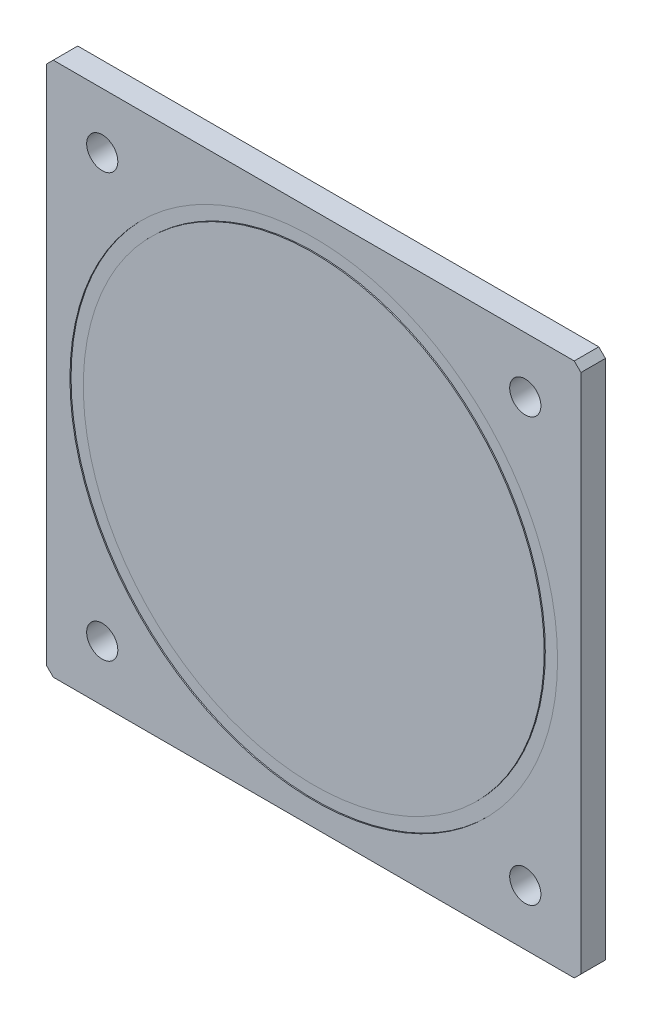
from build123d import *

# Parameters (mm, degrees)
SKETCH1_W           = 240
SKETCH1_H           = 240
BOSS_EXTRUDE1_DEPTH = 11
SKETCH2_R           = 109.5
SKETCH2_R_2         = 103.5
CUT_EXTRUDE1_DEPTH  = 0.5
SKETCH3_R           = 7
CUT_EXTRUDE2_DEPTH  = 59
CHAMFER1_SIZE       = 3


with BuildPart() as part:
    # Sketch1 → Boss-Extrude1 (new body)
    with BuildSketch(Plane.XY):
        Rectangle(SKETCH1_W, SKETCH1_H)
    extrude(amount=BOSS_EXTRUDE1_DEPTH)

    # Sketch2 → Cut-Extrude1 (cut)
    with BuildSketch(Plane.XY.offset(11)):
        Circle(SKETCH2_R)
        Circle(SKETCH2_R_2, mode=Mode.SUBTRACT)
    extrude(amount=-CUT_EXTRUDE1_DEPTH, mode=Mode.SUBTRACT)

    # Sketch3 → Cut-Extrude2 (cut)
    with BuildSketch(Plane.XY.offset(11)):
        with Locations((-95, 95)):
            Circle(SKETCH3_R)
        with Locations((95, 95)):
            Circle(SKETCH3_R)
        with Locations((95, -95)):
            Circle(SKETCH3_R)
        with Locations((-95, -95)):
            Circle(SKETCH3_R)
    extrude(amount=-CUT_EXTRUDE2_DEPTH, mode=Mode.SUBTRACT)

    # Chamfer1
    chamfer1_edges = [part.edges().sort_by_distance(p)[0] for p in [
        (-120, 120, 5.5),
        (120, 120, 5.5),
        (120, -120, 5.5),
        (-120, -120, 5.5),
    ]]
    chamfer(chamfer1_edges, length=CHAMFER1_SIZE)


solid = part.part
